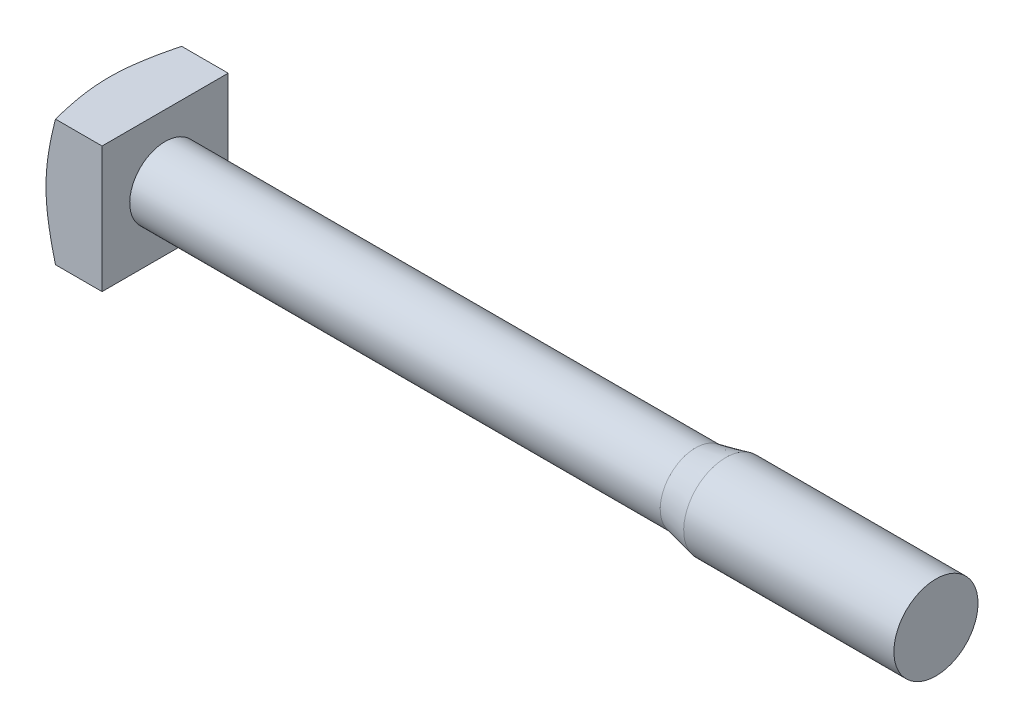
SolidWorks part; units mm, degrees
ref_plane "Front" through (0, 0, 0) normal (0, 0, 1) x (1, 0, 0)
ref_plane "Top" through (0, 0, 0) normal (0, 1, 0) x (1, 0, 0)
ref_plane "Right" through (0, 0, 0) normal (1, 0, 0) x (0, 0, -1)
sketch "Sketch1" plane through (0, 0, 0) normal (1, 0, 0) x (0, 0, -1)
  line L0 (0, 36.5746) -> (0, -34.3123) construction
  line L1 (-37.5173, 0) -> (33.3696, 0) construction
  line L3 (-9, 9) -> (9, 9)
  line L4 (-9, 9) -> (-9, -9)
  line L5 (-9, -9) -> (9, -9)
  line L6 (9, 9) -> (9, -9)
extrude "BaseHead" add sketch "Sketch1" along normal blind 8
ref_plane "Plane1" through (0, 0, 0) normal (0, -0.7071, -0.7071) x (1, 0, 0)
sketch "Sketch4" plane through (-7.1814, -8, 8) normal (0, -0.7071, -0.7071) x (-1, 0, 0)
  line L0 (-16.1283, 11.3137) -> (-5.416, 11.3137) construction
  line L1 (-7.1814, 20.3137) -> (-7.1814, 24.0416)
  line L2 (-7.1814, 24.0416) -> (-8.5383, 24.0416)
  line L3 (-8.5383, 24.0416) -> (-7.1814, 20.3137)
revolve "HeadChamfer" cut sketch "Sketch4" angle 360 about L0
sketch "Sketch2" plane through (8, 0, 0) normal (1, 0, 0) x (0, 0, -1)
  circle A0 centre (0, 0) radius 6
extrude "BaseBody" add sketch "Sketch2" along normal blind 110
cosmetic thread "ThreadCosmetic1" [suppressed] parameters "D2"=10.106
sketch "Sketch5" plane through (-43.2091, 5, 0) normal (0, 0, 1) x (-1, 0, 0)
  line L0 (-39.4181, 5) -> (-75.6573, 5) construction
  line L1 (-131.2091, 11) -> (-51.2091, 11)
  line L2 (-51.2091, 14) -> (-51.2091, -4) construction
  line L4 (-131.2091, 11) -> (-126.9091, 10.053)
  line L5 (-126.9091, 10.053) -> (-51.2091, 10.053)
  line L6 (-161.2091, 11) -> (-161.2091, -1) construction
  line L7 (-51.2091, 11) -> (-51.2091, 10.053)
  line L8 (-51.2091, 11) -> (-161.2091, 11) construction
  dimension "b" = 30
  dimension "dz" = 10.106
  dimension "x" = 4.3
revolve "Cut-Revolve1" cut sketch "Sketch5" angle 360 about L0
sketch "Sketch6" plane through (0, 0, 0) normal (0, 0, 1) x (1, 0, 0)
  line L0 (117.5265, 6.947) -> (118.4735, 6.947)
  line L1 (118.4735, 6.947) -> (118.4735, 6)
  line L2 (118.4735, 6) -> (118, 5.1799)
  line L3 (118, 5.1799) -> (117.5265, 6)
  line L4 (117.5265, 6) -> (117.5265, 6.947)
  line L5 (118, -6) -> (118, 6) construction
  line L8 (0, 0) -> (57.2897, 0) construction
  line L9 (8.9468, 0) -> (-1.7654, 0) construction
revolve "Cut-Revolve10" [suppressed] cut sketch "Sketch6" angle 360
pattern_linear "LPattern10" [suppressed] count 97
equation "\"D2@Sketch4\" = \"s@Sketch1\""
equation "\"D1@Sketch6\" =  ( \"d@Sketch2\" - \"D2@ThreadCosmetic1\" )  / 2"
equation "\"pitch@LPattern10\" = 1.2 * \"D1@Sketch6\""
equation "\"D1@LPattern10\" =  \"l@BaseBody\"  / \"pitch@LPattern10\""
equation "\"D2@Sketch6\" = \"d@Sketch2\""
